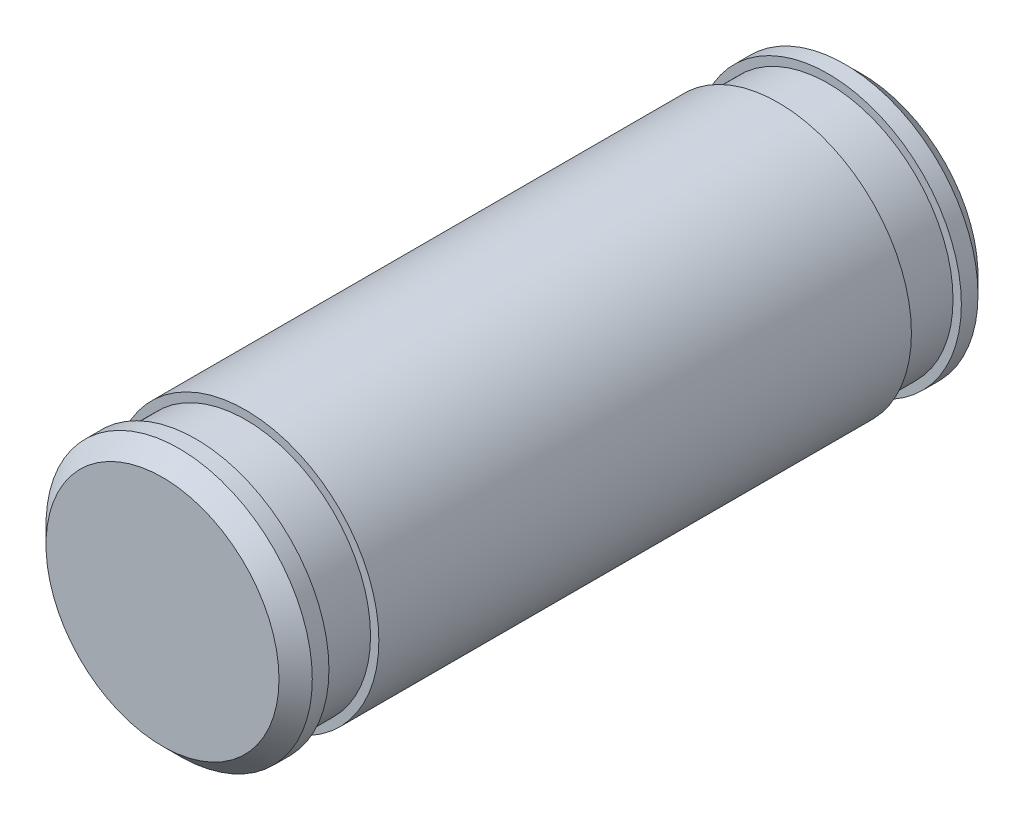
from build123d import *

# Parameters (mm, degrees)
SKETCH1_R                = 4
BOSS_EXTRUDE1_DEPTH      = 8
SKETCH2_R                = 3.75
BOSS_EXTRUDE2_DEPTH      = 1.5
BOSS_EXTRUDE3_START      = 1
SKETCH3_R                = 4
BOSS_EXTRUDE3_DEPTH      = 1
CHAMFER1_SIZE            = 0.5
CHAMFER1_OF_MIRROR1_SIZE = 0.5


with BuildPart() as part:
    # Sketch1 → Boss-Extrude1 (new, symmetric)
    with BuildSketch(Plane.XY):
        Circle(SKETCH1_R)
    extrude(amount=BOSS_EXTRUDE1_DEPTH, both=True)

    # Sketch2 → Boss-Extrude2 (add)
    with BuildSketch(Plane.XY.offset(8)):
        Circle(SKETCH2_R)
    boss_extrude2 = extrude(amount=BOSS_EXTRUDE2_DEPTH)

    # Sketch3 → Boss-Extrude3 (add)
    with BuildSketch(Plane.XY.offset(9.5).offset(BOSS_EXTRUDE3_START)):
        Circle(SKETCH3_R)
    boss_extrude3 = extrude(amount=-BOSS_EXTRUDE3_DEPTH)

    # Chamfer1
    chamfer1_edges = [part.edges().sort_by_distance(p)[0] for p in [
        (-4, 0, 10.5),
    ]]
    chamfer(chamfer1_edges, length=CHAMFER1_SIZE)

    # Mirror1: Boss-Extrude2, Boss-Extrude3 across plane
    add(boss_extrude2.mirror(Plane.XY))
    add(boss_extrude3.mirror(Plane.XY))

    # Chamfer1 of Mirror1
    chamfer1_of_mirror1_edges = [part.edges().sort_by_distance(p)[0] for p in [
        (-4, 0, -10.5),
    ]]
    chamfer(chamfer1_of_mirror1_edges, length=CHAMFER1_OF_MIRROR1_SIZE)


solid = part.part
